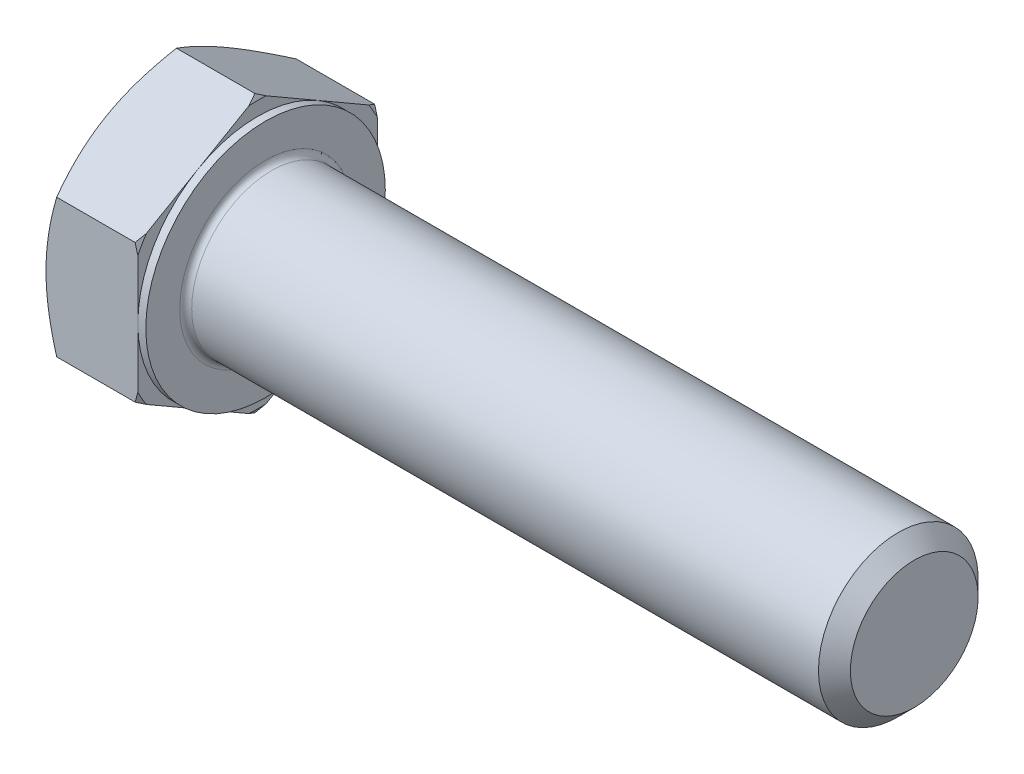
SolidWorks part; units mm, degrees
extrude "基体-拉伸" add sketch "草图1" along normal blind 10
sketch "草图1" plane through (0, 0, 0) normal (1, 0, 0) x (0, 0, -1)
  line L0 (12, 6.9282) -> (12, -6.9282)
  line L1 (-12, 6.9282) -> (-12, -6.9282)
  line L2 (12, -6.9282) -> (0, -13.8564)
  line L3 (0, -13.8564) -> (-12, -6.9282)
  line L4 (12, 6.9282) -> (0, 13.8564)
  line L5 (0, 13.8564) -> (-12, 6.9282)
revolve "切除-旋转1" cut sketch "草图3" angle 360 about L6
sketch "草图3" plane through (0, 0, 0) normal (0, 0, 1) x (1, 0, 0)
  line L0 (0, 12) -> (3.9585, 18.8564)
  line L1 (0, 13.8564) -> (0, 6.9282) construction
  line L2 (3.9585, 18.8564) -> (3.9585, 23.8564)
  line L3 (3.9585, 23.8564) -> (-10, 23.8564)
  line L4 (-10, 23.8564) -> (-10, 12)
  line L5 (-10, 12) -> (0, 12)
  line L6 (0, 0) -> (99.06, 0) construction
  line L7 (10, 13.8564) -> (0, 13.8564) construction
material "5.6级"
ref_plane "前视" through (0, 0, 0) normal (0, 0, 1) x (1, 0, 0)
ref_plane "上视" through (0, 0, 0) normal (0, 1, 0) x (1, 0, 0)
ref_plane "右视" through (0, 0, 0) normal (1, 0, 0) x (0, 0, -1)
sketch "草图2" plane through (0, 0, 0) normal (0, 0, 1) x (1, 0, 0)
  line L0 (0, 6.9282) -> (0, -6.9282) construction
  line L1 (0, 0) -> (75, 0)
  line L2 (0, 0) -> (0, 8)
  line L3 (0, 8) -> (7.7917, 8)
  line L4 (75, 0) -> (75, 6.268)
  line L5 (10, 13.8564) -> (10, 6.9282) construction
  line L7 (0, 0) -> (96.52, 0) construction
  line L8 (75, -6.268) -> (7.7917, -8) construction
  line L9 (0, -8) -> (7.7917, -8) construction
  line L10 (12, 15.24) -> (12, -1.27) construction
  line L11 (37, 15.24) -> (37, -1.27) construction
  line L12 (10, 6.9282) -> (10, -6.9282) construction
  line L13 (7.7917, 8) -> (75, 8)
  line L14 (75, 8) -> (75, 6.268)
revolve "凸台-旋转1" add sketch "草图2" angle 360 about L7
cosmetic thread "螺旋线1" parameters "Thread_length"=38, "Thread_minor"=12.536
sketch "草图5" plane through (0, 0, 0) normal (0, 0, 1) x (1, 0, 0)
  line L0 (10, 12) -> (6.0415, 18.8564)
  line L1 (10, 13.8564) -> (10, 6.9282) construction
  line L2 (6.0415, 18.8564) -> (6.0415, 23.8564)
  line L3 (6.0415, 23.8564) -> (16.0415, 23.8564)
  line L4 (16.0415, 23.8564) -> (16.0415, 12)
  line L5 (16.0415, 12) -> (10, 12)
  line L7 (10, 13.8564) -> (1.0718, 13.8564) construction
  line L8 (0, 0) -> (99.06, 0) construction
  line L9 (0, 0) -> (99.06, 0) construction
revolve "切除-旋转2" cut sketch "草图5" angle 360 about L8
sketch "草图4" plane through (0, 0, 0) normal (0, 0, 1) x (1, 0, 0)
  line L1 (10, 13.8564) -> (10, 6.9282) construction
  line L2 (10, 12) -> (9.2, 12)
  line L3 (10, 12) -> (10, 23.8564)
  line L4 (10, 23.8564) -> (9.2, 23.8564)
  line L5 (0, 0) -> (95.25, 0) construction
  line L6 (0, 0) -> (96.52, 0) construction
  line L7 (9.2, 12) -> (9.2, 23.8564)
  line L8 (8.9282, 13.8564) -> (1.0718, 13.8564) construction
revolve "切除-旋转3" cut sketch "草图4" angle 360 about L5
chamfer "倒角" distance 1.6 angle 45 1 edges at (75, 0, 8)
fillet "圆角" radius 0.6 1 edges at (10, 0, -8)
sketch "草图6" plane through (0, 0, 0) normal (0, 0, 1) x (1, 0, 0)
  line L0 (37, -6.268) -> (36, -8)
  line L1 (37, -6.268) -> (38, -8)
  line L2 (38, -8) -> (38, -10)
  line L3 (-3.175, 0) -> (5.1513, 0) construction
  line L5 (38, -10) -> (36, -10)
  line L6 (36, -10) -> (36, -8)
revolve "切除-旋转4" [suppressed] cut sketch "草图6" angle 360 about L3
pattern_linear "阵列(线性)1" [suppressed]
equation "\"D3@草图1\" = \"s@草图1\" / 2"
equation "\"D4@草图1\" = \"D3@草图1\""
equation "\"D5@草图1\" = \"D4@草图1\""
equation "\"Thread_minor@螺旋线1\" = \"Minor_dia@草图2\""
equation "\"D1@草图3\" = \"s@草图1\" / 2"
equation "\"D1@草图5\" = \"s@草图1\" / 2"
equation "\"Head_ch_ang@草图5\" = \"Head_ch_ang@草图3\""
equation "\"D1@草图4\" = \"s@草图1\""
equation "\"Thread_length@螺旋线1\" = ((sgn( (\"l@草图2\" - \"p@草图2\" ) - \"h@草图2\" )-1)*( (\"l@草图2\" - \"p@草图2\" ) - \"h@草图2\" ))/-2+ \"h@草图2\""
equation "\"Thread_minor@草图6\" = \"Minor_dia@草图2\""
equation "\"Diameter@草图6\" = \"m@草图2\""
equation "\"Overcut@草图6\" = \"m@草图2\" * 1.25"
equation "\"Start@草图6\" = \"k@基体-拉伸\" + \"l@草图2\" - \"Thread_length@螺旋线1\"  '---Non-countersunk---"
equation "\"Num_threads@阵列(线性)1\" = int( \"Thread_length@螺旋线1\" / \"p@草图2\" + 0.999 )  + 1"
equation "\"Advance@阵列(线性)1\" = \"Thread_length@螺旋线1\" /  (\"Num_threads@阵列(线性)1\" - 1) 'relax it"
equation "\"Num_threads@阵列(线性)1\" = \"Num_threads@阵列(线性)1\" - sgn( \"Num_threads@阵列(线性)1\" - 1) '---chamfered tips only---"
equation "\"Minor_dia@草图2\" = \"m@草图2\"-\"p@草图2\" * 1.732"
equation "\"D1@倒角\" = \"p@草图2\"*0.8"
